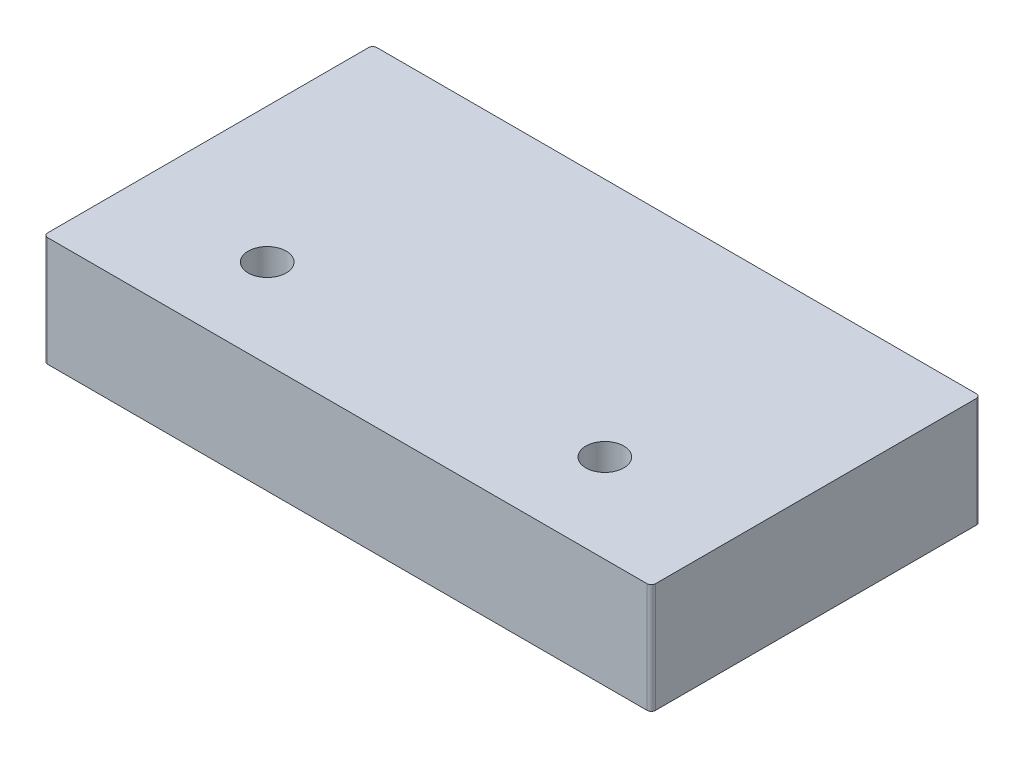
from build123d import *

# Parameters (mm, degrees)
SKETCH_1_W          = 72
SKETCH_1_H          = 13
EXTRUDE_1_DEPTH     = 39
FILLET_1_R          = 0.5
SKETCH_2_R          = 2.25
CUT_EXTRUDE_1_DEPTH = 55.644304369


with BuildPart() as part:
    # 草图1 → 凸台-拉伸1 (new body)
    with BuildSketch(Plane.XY):
        Rectangle(SKETCH_1_W, SKETCH_1_H)
    extrude(amount=EXTRUDE_1_DEPTH)

    # 圆角1
    fillet_1_edges = [part.edges().sort_by_distance(p)[0] for p in [
        (36, 0, 39),
        (-36, 0, 39),
        (36, 0, 0),
        (-36, 0, 0),
    ]]
    fillet(fillet_1_edges, radius=FILLET_1_R)

    # 草图2 → 切除-拉伸1 (cut, through all)
    with BuildSketch(Plane(origin=(0, 6.5, 0), x_dir=(1, 0, 0), z_dir=(0, 1, 0))):
        with Locations(Location((-20, -28.5, 0), (0, 0, 180))):
            Circle(SKETCH_2_R)
        with Locations(Location((20, -28.5, 0), (0, 0, 180))):
            Circle(SKETCH_2_R)
    extrude(amount=-CUT_EXTRUDE_1_DEPTH, mode=Mode.SUBTRACT)


solid = part.part
